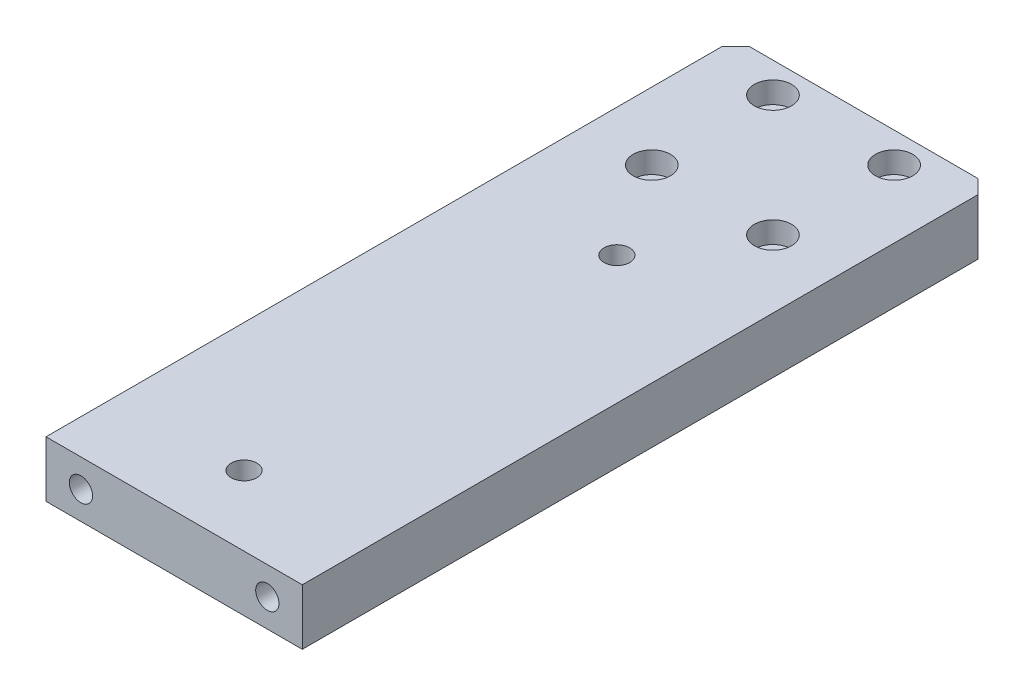
SolidWorks part; units mm, degrees
material "A6061"
ref_plane "前基準面" through (0, 0, 0) normal (0, 0, 1) x (1, 0, 0)
ref_plane "上基準面" through (0, 0, 0) normal (0, 1, 0) x (1, 0, 0)
ref_plane "右基準面" through (0, 0, 0) normal (1, 0, 0) x (0, 0, -1)
sketch "草图1" plane through (0, 0, 0) normal (0, 1, 0) x (1, 0, 0)
  line L1 (-27.5, -74) -> (27.5, -74)
  line L2 (-27.5, -74) -> (-27.5, 74)
  line L3 (-27.5, 74) -> (27.5, 74)
  line L4 (27.5, -74) -> (27.5, 74)
  line L5 (-27.5, -74) -> (27.5, 74) construction
  line L6 (-27.5, 74) -> (27.5, -74) construction
  point P0 (0, 0)
  dimension "D1" = 55
  dimension "D2" = 148
extrude "凸台-拉伸1" add sketch "草图1" along normal mid plane 12
chamfer "倒角1" distance 3 angle 45 2 edges at (-27.5, 0, -74) (27.5, 0, -74)
hole_wizard "打孔尺寸(%根据)内六角圆柱头螺钉的类型1" positions "草图2" profile "草图3" counterbore size "M4" standard "GB" end condition through all
sketch "草图2" plane through (0, 6, 0) normal (0, 1, 0) x (1, 0, 0)
  line L0 (0, 0) -> (0, 84.2019) construction
  line L2 (-27.5, -74) -> (27.5, -74) construction
  point P0 (13, 41.5)
  point P2 (13, 67.5)
  point P10 (-13, 67.5)
  point P11 (-13, 41.5)
  dimension "D1" = 26
  dimension "D2" = 26
  dimension "D3" = 115.5
sketch "草图3" plane through (13, 6, -41.5) normal (1, 0, 0) x (0, 0, 1)
  line L0 (0, 0) -> (0, 12)
  line L1 (0, 12) -> (2.25, 12)
  line L3 (2.25, 12) -> (2.25, 4.6)
  line L4 (2.25, 4.6) -> (4, 4.6)
  line L5 (4, 4.6) -> (4, 0)
  line L7 (4, 0) -> (0, 0)
  line L11 (0, -6.35) -> (0, 107.95) construction
  dimension "通孔孔直径" = 4.5
  dimension "通孔孔深度" = 12
  dimension "柱形沉头孔直径" = 8
  dimension "柱形沉头孔深度" = 4.6
hole_wizard "M6 螺纹孔1" positions "草图4" profile "草图5" tap size "M6" standard "GB"
sketch "草图4" plane through (0, 0, 74) normal (0, 0, 1) x (1, 0, 0)
  line L0 (0, -9.9396) -> (0, 0) construction
  point P0 (20, 0)
  point P12 (-20, 0)
  dimension "D1" = 40
sketch "草图5" plane through (20, 0, 74) normal (1, 0, 0) x (0, -1, 0)
  line L0 (0, 0) -> (0, 16.5022)
  line L1 (0, 16.5022) -> (2.5, 15)
  line L2 (2.5, 15) -> (2.5, 0)
  line L5 (2.5, 0) -> (0, 0)
  line L10 (0, 16.5022) -> (-2.5, 15) construction
  line L11 (0, -6.35) -> (0, 107.95) construction
  dimension "螺纹孔钻头直径" = 5
  dimension "螺纹孔钻头深度" = 15
  dimension "导头角度" = 118
cosmetic thread "孔螺蚊线1" parameters "D1"=12, "D2"=6
cosmetic thread "孔螺蚊线2" parameters "D1"=12, "D2"=6
hole_wizard "打孔尺寸(%根据)内六角圆柱头螺钉的类型2" positions "草图6" profile "草图7" counterbore size "M5" standard "GB" end condition through all
sketch "草图6" plane through (0, -6, 0) normal (0, 1, 0) x (1, 0, 0)
  line L0 (-27.5, -74) -> (27.5, -74) construction
  point P0 (0, -59)
  point P2 (0, 21)
  dimension "D1" = 15
  dimension "D2" = 80
sketch "草图7" plane through (0, -6, 59) normal (1, 0, 0) x (0, 0, -1)
  line L0 (0, 0) -> (0, 12)
  line L1 (0, 12) -> (2.75, 12)
  line L3 (2.75, 12) -> (2.75, 5.7)
  line L4 (2.75, 5.7) -> (5, 5.7)
  line L5 (5, 5.7) -> (5, 0)
  line L7 (5, 0) -> (0, 0)
  line L11 (0, -6.35) -> (0, 107.95) construction
  dimension "通孔孔直径" = 5.5
  dimension "通孔孔深度" = 12
  dimension "柱形沉头孔直径" = 10
  dimension "柱形沉头孔深度" = 5.7
